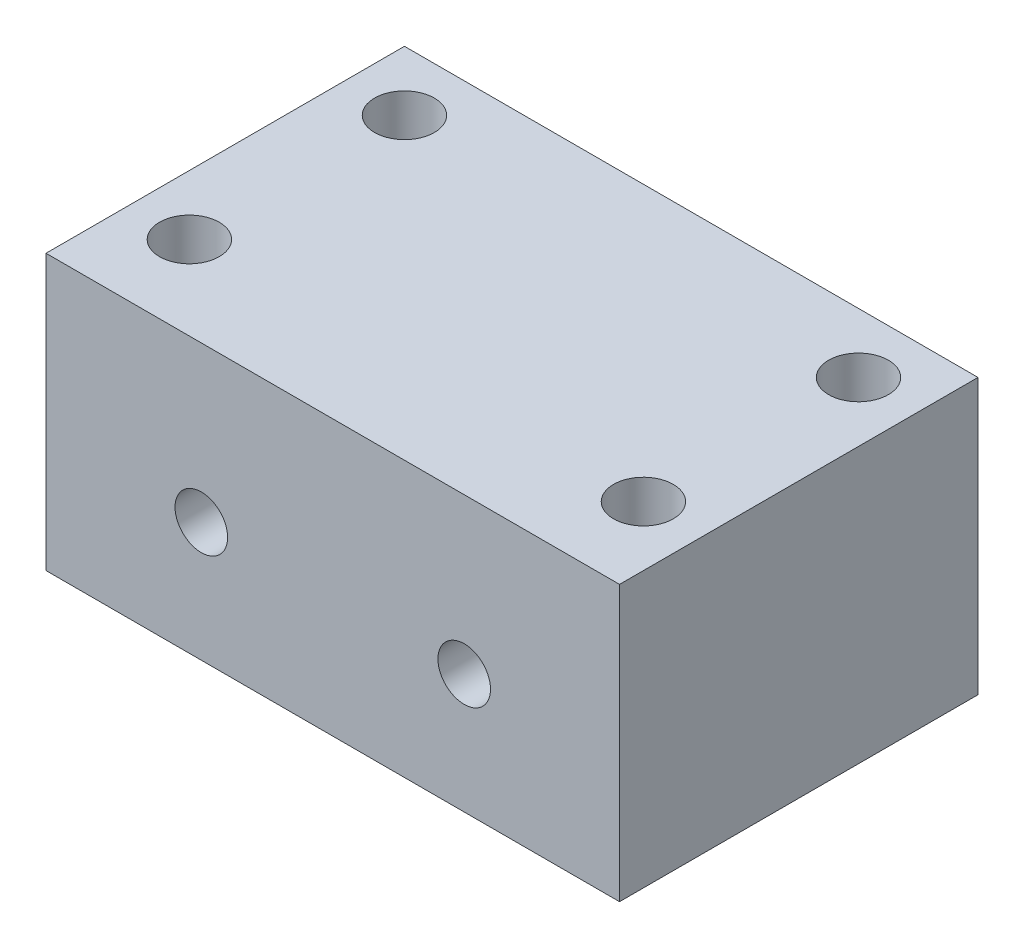
SolidWorks part; units mm, degrees
ref_plane "前视基准面" through (0, 0, 0) normal (0, 0, 1) x (1, 0, 0)
ref_plane "上视基准面" through (0, 0, 0) normal (0, 1, 0) x (1, 0, 0)
ref_plane "右视基准面" through (0, 0, 0) normal (1, 0, 0) x (0, 0, -1)
sketch "草图1" plane through (0, 0, 0) normal (0, 0, 1) x (1, 0, 0)
  line L1 (-24.5455, 16.5273) -> (23.4545, 16.5273)
  line L2 (-24.5455, 16.5273) -> (-24.5455, -13.4727)
  line L3 (-24.5455, -13.4727) -> (23.4545, -13.4727)
  line L4 (23.4545, 16.5273) -> (23.4545, -13.4727)
  dimension "D1" = 48
  dimension "D2" = 30
extrude "凸台-拉伸1" add sketch "草图1" along normal blind 30
sketch "草图2" plane through (0, 0, 0) normal (0, 0, -1) x (-1, 0, 0)
  line L0 (24.5455, -13.4727) -> (-23.4545, -13.4727) construction
  line L1 (-13.4545, -13.4727) -> (14.5455, -13.4727)
  line L2 (-13.4545, -13.4727) -> (-13.4545, 1.5273)
  line L3 (-13.4545, 1.5273) -> (14.5455, 1.5273)
  line L4 (14.5455, -13.4727) -> (14.5455, 1.5273)
  line L5 (-23.4545, -13.4727) -> (-23.4545, 16.5273) construction
  dimension "D1" = 28
  dimension "D2" = 15
  dimension "D3" = 10
extrude "切除-拉伸1" cut sketch "草图2" against normal blind 20
sketch "草图3" plane through (0, 0, 20) normal (0, 0, -1) x (-1, 0, 0)
  line L0 (14.5455, 1.5273) -> (-13.4545, 1.5273) construction
  line L1 (-13.4545, 1.5273) -> (-13.4545, -13.4727) construction
  line L2 (14.5455, 1.5273) -> (-13.4545, 1.5273) construction
  line L3 (14.5455, -13.4727) -> (14.5455, 1.5273) construction
  circle A0 centre (-10.4545, -3.4727) radius 2.2
  circle A1 centre (11.5455, -3.4727) radius 2.2
  dimension "D5" = 4.4
  dimension "D6" = 4.4
  dimension "D1" = 5
  dimension "D2" = 3
  dimension "D3" = 5
  dimension "D4" = 3
extrude "切除-拉伸2" cut sketch "草图3" against normal blind 20
sketch "草图4" plane through (0, -13.4727, 0) normal (0, -1, 0) x (1, 0, 0)
  line L0 (-24.5455, 30) -> (23.4545, 30) construction
  line L1 (-24.5455, 30) -> (-24.5455, 0) construction
  line L2 (-24.5455, 0) -> (-14.5455, 0) construction
  line L3 (23.4545, 30) -> (23.4545, 0) construction
  line L4 (13.4545, 0) -> (23.4545, 0) construction
  circle A1 centre (-19.5455, 5) radius 2.5
  circle A2 centre (-19.5455, 23) radius 2.5
  circle A3 centre (18.4545, 23) radius 2.5
  circle A4 centre (18.4545, 5) radius 2.5
  dimension "D9" = 5
  dimension "D10" = 5
  dimension "D11" = 5
  dimension "D12" = 5
  dimension "D1" = 7
  dimension "D2" = 5
  dimension "D3" = 5
  dimension "D4" = 5
  dimension "D5" = 5
  dimension "D6" = 5
  dimension "D7" = 5
  dimension "D8" = 7
extrude "切除-拉伸3" cut sketch "草图4" against normal up to surface (30 mm away) up to face at (-0.5455, 16.5273, 15)
sketch "草图8" plane through (0, 0, 30) normal (0, 0, 1) x (1, 0, 0)
  line L0 (-24.5455, 16.5273) -> (-24.5455, -13.4727) construction
  line L1 (23.4545, 16.5273) -> (-24.5455, 16.5273)
  line L2 (23.4545, 16.5273) -> (23.4545, 9.5273)
  line L3 (23.4545, 9.5273) -> (-24.5455, 9.5273)
  line L4 (-24.5455, 16.5273) -> (-24.5455, 9.5273)
  dimension "D1" = 7
extrude "切除-拉伸5" cut sketch "草图8" against normal up to surface (30 mm away)
